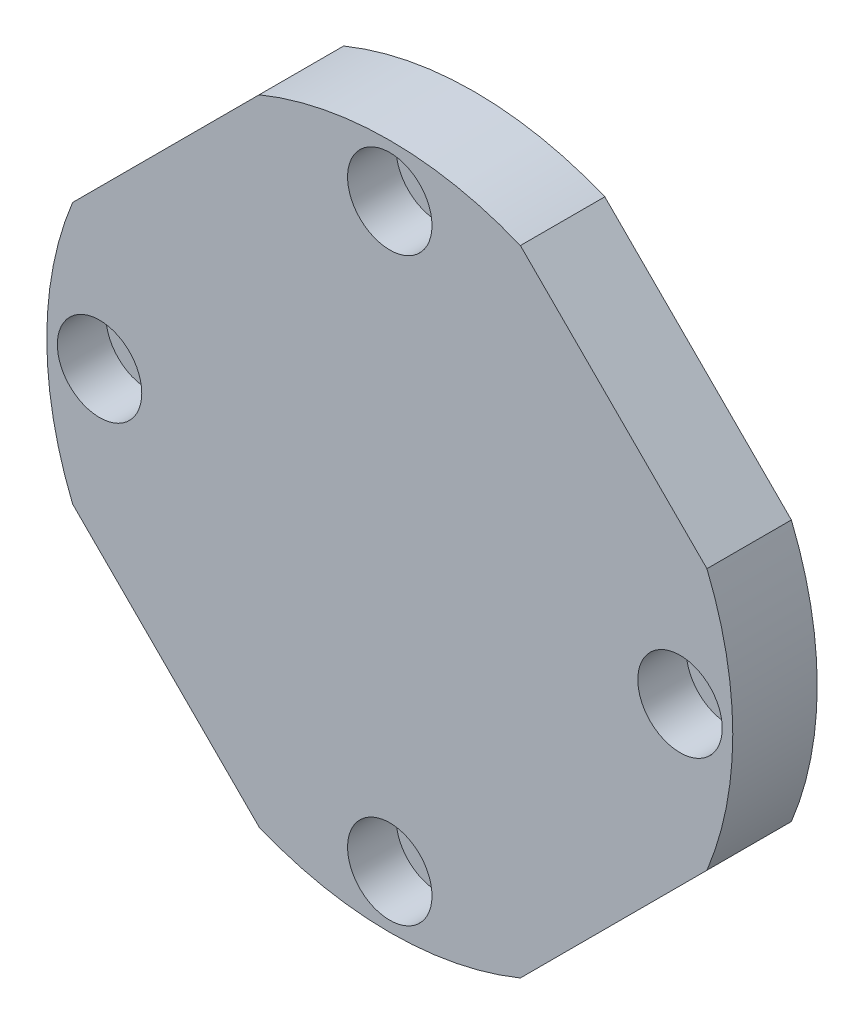
SolidWorks part; units mm, degrees
ref_plane "Front Plane" through (0, 0, 0) normal (0, 0, 1) x (1, 0, 0)
ref_plane "Top Plane" through (0, 0, 0) normal (0, 1, 0) x (1, 0, 0)
ref_plane "Right Plane" through (0, 0, 0) normal (1, 0, 0) x (0, 0, -1)
sketch "Sketch1" plane through (0, 0, 0) normal (0, 0, 1) x (1, 0, 0)
  line L0 (-30.052, -12.3744) -> (-12.3744, -30.052)
  line L1 (-30.052, 12.3744) -> (-12.3744, 30.052)
  line L2 (12.3744, -30.052) -> (30.052, -12.3744)
  line L3 (12.3744, 30.052) -> (30.052, 12.3744)
  arc A0 (-30.052, 12.3744) -> (-30.052, -12.3744) centre (0, 0) ccw
  arc A1 (-12.3744, -30.052) -> (12.3744, -30.052) centre (0, 0) ccw
  arc A2 (30.052, -12.3744) -> (30.052, 12.3744) centre (0, 0) ccw
  arc A3 (12.3744, 30.052) -> (-12.3744, 30.052) centre (0, 0) ccw
  dimension "D1" = 65
extrude "Boss-Extrude1" add sketch "Sketch1" along normal blind 8
hole_wizard "Hole size per socket head cap screw type 1" positions "Sketch3" profile "Sketch2" counterbore size "M4" standard "GB" end condition through all
sketch "Sketch3" plane through (0, 0, 8) normal (0, 0, 1) x (1, 0, 0)
  circle A0 centre (0, 0) radius 27.5 construction
  point P0 (0, 27.5)
  point P1 (-27.5, 0)
  point P3 (0, -27.5)
  point P5 (27.5, 0)
  dimension "D1" = 55
sketch "Sketch2" plane through (0, 27.5, 8) normal (1, 0, 0) x (0, -1, 0)
  line L0 (0, 0) -> (0, 8)
  line L1 (0, 8) -> (2.25, 8)
  line L3 (2.25, 8) -> (2.25, 4.6)
  line L4 (2.25, 4.6) -> (4, 4.6)
  line L5 (4, 4.6) -> (4, 0)
  line L7 (4, 0) -> (0, 0)
  line L11 (0, -6.35) -> (0, 107.95) construction
  dimension "通孔孔直径" = 4.5
  dimension "通孔孔深度" = 8
  dimension "柱形沉头孔直径" = 8
  dimension "柱形沉头孔深度" = 4.6
